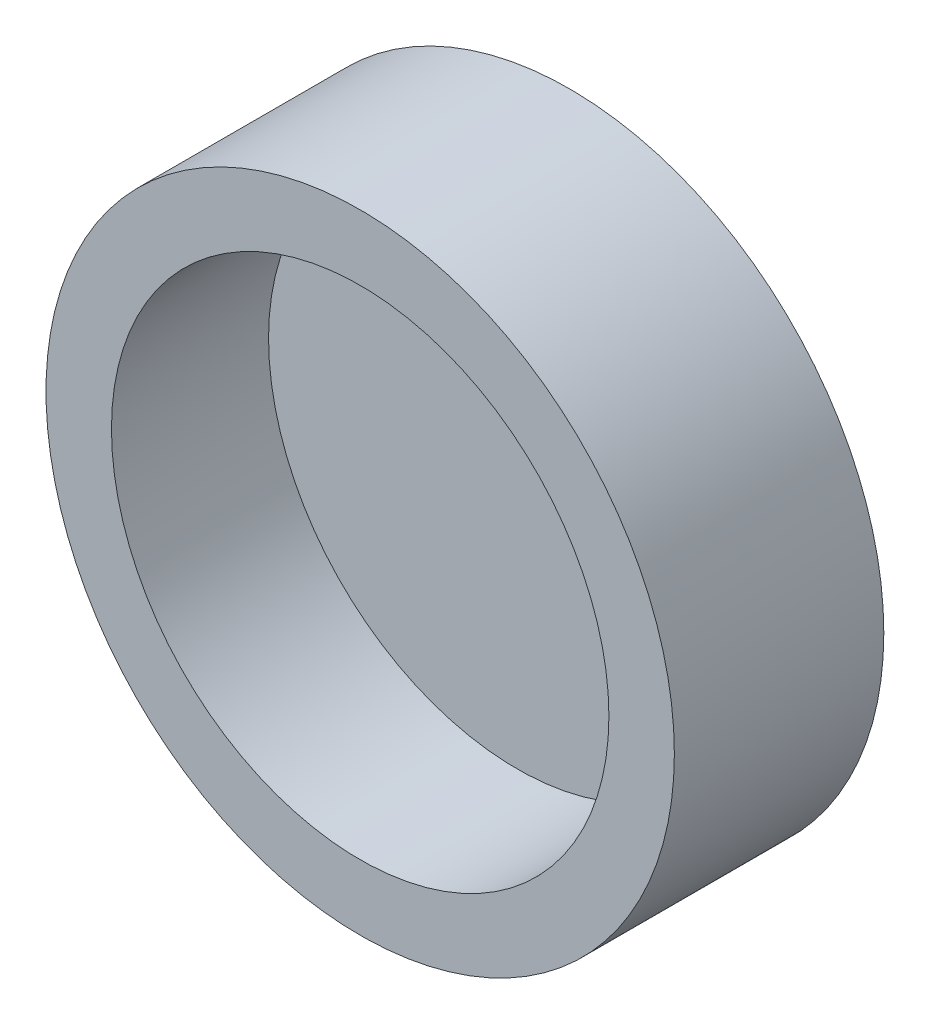
SolidWorks part; units mm, degrees
ref_plane "Front Plane" through (0, 0, 0) normal (0, 0, 1) x (1, 0, 0)
ref_plane "Top Plane" through (0, 0, 0) normal (0, 1, 0) x (1, 0, 0)
ref_plane "Right Plane" through (0, 0, 0) normal (1, 0, 0) x (0, 0, -1)
sketch "Sketch1" plane through (0, 0, 0) normal (0, 0, 1) x (1, 0, 0)
  circle A0 centre (0, 0) radius 12
extrude "Boss-Extrude1" add sketch "Sketch1" along normal blind 8
sketch "Sketch2" plane through (0, 0, 8) normal (0, 0, 1) x (1, 0, 0)
  circle A0 centre (0, 0) radius 9.5
  dimension "D1" = 19
extrude "Cut-Extrude1" cut sketch "Sketch2" against normal blind 6
